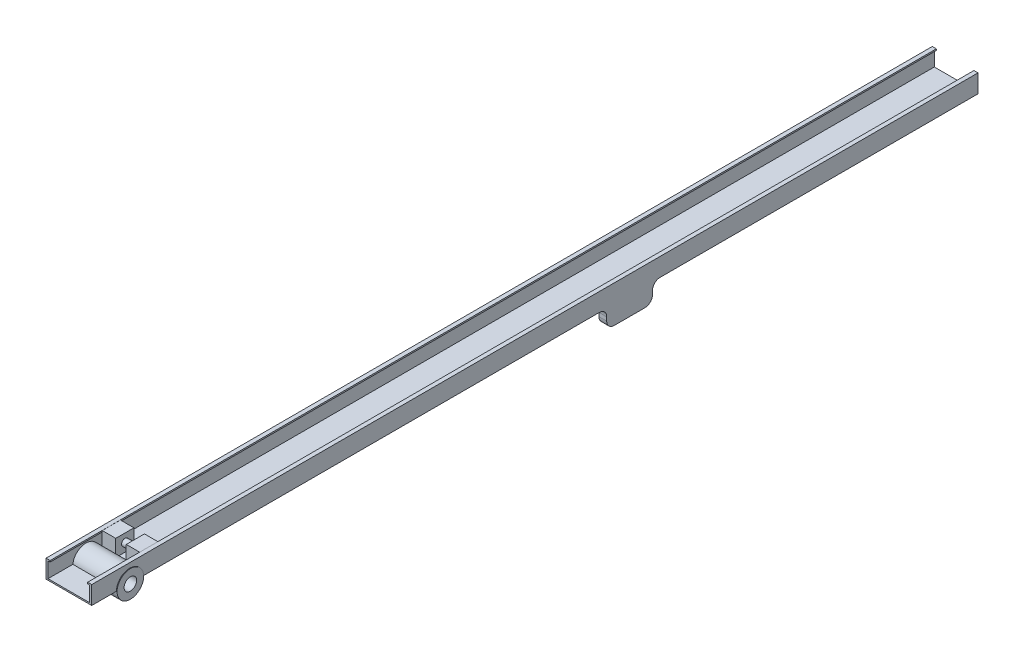
from build123d import *

# Parameters (mm, degrees)
BOSS_EXTRUDE1_DEPTH     = 7075
SKETCH4_W               = 730
SKETCH4_H               = 731.509808534
BOSS_EXTRUDE2_DEPTH     = 299
FILLET1_R               = 120
FILLET2_R               = 120
SKETCH7_R               = 212.119628044
BOSS_EXTRUDE3_DEPTH     = 375
SKETCH8_R               = 87.5
BOSS_EXTRUDE4_DEPTH     = 425
CUT_EXTRUDE1_DEPTH      = 194
CUT_EXTRUDE1_DEPTH_BACK = 930
SKETCH9_W               = 484.11997185
SKETCH9_H               = 481.593519394
SKETCH12_R              = 85
BOSS_EXTRUDE5_DEPTH     = 548
SKETCH14_R              = 90
BOSS_EXTRUDE6_DEPTH     = 167.01
BOSS_EXTRUDE7_START     = 167.01
SKETCH15_R              = 90
BOSS_EXTRUDE7_DEPTH     = 167.01
SKETCH16_W              = 216
SKETCH16_H              = 290.579133159
BOSS_EXTRUDE8_DEPTH     = 266
SKETCH17_R              = 55
BOSS_EXTRUDE9_DEPTH     = 238
SKETCH18_R              = 87.5
CUT_EXTRUDE2_DEPTH      = 7140.696141994
SKETCH19_R              = 100
CUT_EXTRUDE3_DEPTH      = 7129.482377056


with BuildPart() as part:
    # Sketch1 → Boss-Extrude1 (new, symmetric)
    with BuildSketch(Plane.XY):
        Polygon((-300, 145), (-300, 122.5), (-332.5, 122.5), (-332.5, -122.5), (332.5, -122.5), (332.5, 122.5), (300, 122.5), (300, 145), (365, 145), (365, -145), (-365, -145), (-365, 145), align=None)
    extrude(amount=BOSS_EXTRUDE1_DEPTH, both=True)

    # Sketch4 → Boss-Extrude2 (add)
    with BuildSketch(Plane.XZ.offset(145)):
        with Locations((0, -1512.728660923)):
            Rectangle(SKETCH4_W, SKETCH4_H)
    extrude(amount=BOSS_EXTRUDE2_DEPTH)

    # Fillet1
    fillet1_edges = [part.edges().sort_by_distance(p)[0] for p in [
        (0, -444, -1146.973756656),
        (0, -444, -1878.48356519),
    ]]
    fillet(fillet1_edges, radius=FILLET1_R)

    # Fillet2
    fillet2_edges = [part.edges().sort_by_distance(p)[0] for p in [
        (0, -145, -1146.973756656),
        (0, -145, -1878.48356519),
    ]]
    fillet(fillet2_edges, radius=FILLET2_R)

    # Sketch7 → Boss-Extrude3 (add, symmetric)
    with BuildSketch(Plane(origin=(0, 0, 0), x_dir=(0, 0, -1), z_dir=(1, 0, 0))):
        with Locations((-6467.996106232, -145)):
            Circle(SKETCH7_R)
    extrude(amount=BOSS_EXTRUDE3_DEPTH, both=True)

    # Sketch8 → Boss-Extrude4 (add, symmetric)
    with BuildSketch(Plane(origin=(0, 0, 0), x_dir=(0, 0, -1), z_dir=(1, 0, 0))):
        with Locations((-6467.996106232, -145)):
            Circle(SKETCH8_R)
    extrude(amount=BOSS_EXTRUDE4_DEPTH, both=True)

    # Sketch9 → Cut-Extrude1 (cut, two sides: drawn at the far end of the back side and taken through both)
    with BuildSketch(Plane.XY.offset(-1146.973756656).offset(-CUT_EXTRUDE1_DEPTH_BACK)):
        with Locations((0, -381.996563184)):
            Rectangle(SKETCH9_W, SKETCH9_H)
    extrude(amount=CUT_EXTRUDE1_DEPTH + CUT_EXTRUDE1_DEPTH_BACK, mode=Mode.SUBTRACT)

    # Sketch12 → Boss-Extrude5 (add)
    with BuildSketch(Plane.ZY.offset(-242.059985925)):
        with Locations(Location((-1512.728660923, -294, 0), (0, 0, 180))):
            Circle(SKETCH12_R)
    extrude(amount=BOSS_EXTRUDE5_DEPTH)

    # Sketch14 → Boss-Extrude6 (add)
    with BuildSketch(Plane.ZY.offset(-242.059985925)):
        with Locations((-1512.728660923, -294)):
            Circle(SKETCH14_R)
    extrude(amount=BOSS_EXTRUDE6_DEPTH)

    # Sketch15 → Boss-Extrude7 (add)
    with BuildSketch(Plane(origin=(-242.059985925, 0, 0), x_dir=(0, 0, -1), z_dir=(1, 0, 0)).offset(BOSS_EXTRUDE7_START)):
        with Locations(Location((1512.728660923, -294, 0), (0, 0, 180))):
            Circle(SKETCH15_R)
    extrude(amount=-BOSS_EXTRUDE7_DEPTH)

    # Sketch16 → Boss-Extrude8 (add)
    with BuildSketch(Plane(origin=(0, -122.5, 0), x_dir=(1, 0, 0), z_dir=(0, 1, 0))):
        with Locations((192, -6097.467973851)):
            Rectangle(SKETCH16_W, SKETCH16_H)
        with Locations((-192, -6097.467973851)):
            Rectangle(SKETCH16_W, SKETCH16_H)
    extrude(amount=BOSS_EXTRUDE8_DEPTH)

    # Sketch17 → Boss-Extrude9 (add)
    with BuildSketch(Plane.ZY.offset(-84)):
        with Locations(Location((6094.796866122, 15.549991037, 0), (0, 0, 90))):
            Circle(SKETCH17_R)
    extrude(amount=BOSS_EXTRUDE9_DEPTH)

    # Sketch18 → Cut-Extrude2 (cut, through all)
    with BuildSketch(Plane(origin=(425, 0, 0), x_dir=(0, 0, -1), z_dir=(1, 0, 0))):
        with Locations((-6467.996106232, -145)):
            Circle(SKETCH18_R)
    extrude(amount=-CUT_EXTRUDE2_DEPTH, mode=Mode.SUBTRACT)

    # Sketch19 → Cut-Extrude3 (cut, through all)
    with BuildSketch(Plane(origin=(375, 0, 0), x_dir=(0, 0, -1), z_dir=(1, 0, 0))):
        with Locations((-6467.996106232, -145)):
            Circle(SKETCH19_R)
    extrude(amount=-CUT_EXTRUDE3_DEPTH, mode=Mode.SUBTRACT)


solid = part.part
